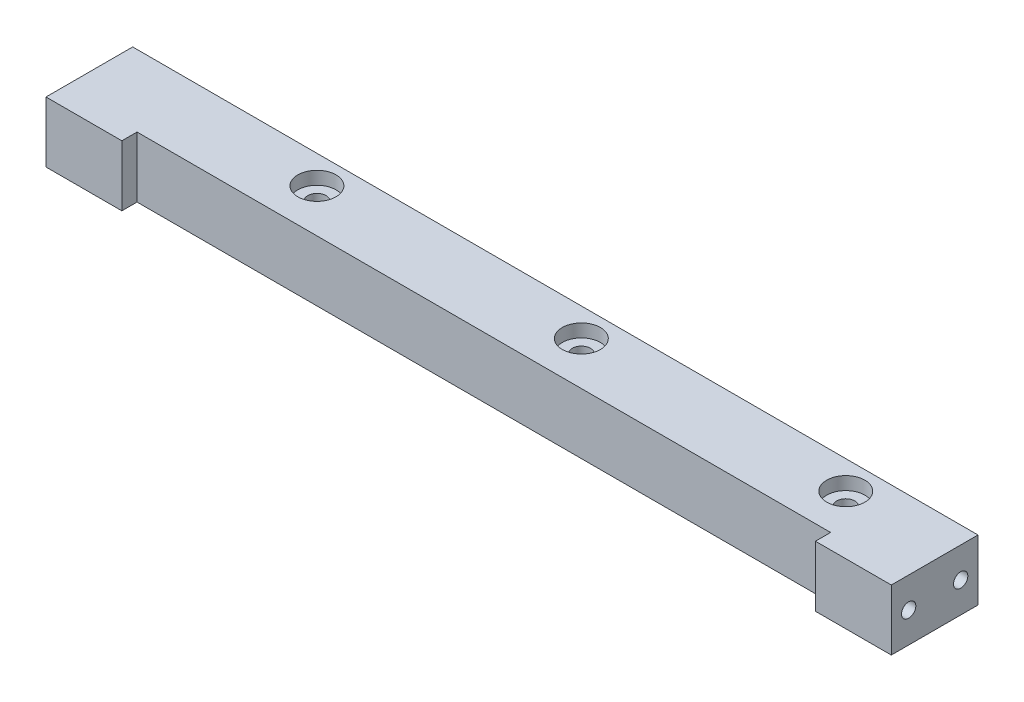
from build123d import *

# Parameters (mm, degrees)
SKETCH1_W             = 195
SKETCH1_H             = 14
EXTRUDE_THIN1_DEPTH   = 10
M4_TAPPED_HOLE1_D     = 3.3
M4_TAPPED_HOLE1_DEPTH = 10.1
M4_TAPPED_HOLE1_TIP   = 0.991420021
M4_TAPPED_HOLE2_D     = 3.3
M4_TAPPED_HOLE2_DEPTH = 10.1
M4_TAPPED_HOLE2_TIP   = 0.991420021
M5_TAPPED_HOLE1_D     = 4.2
SKETCH9_R             = 4.4
CUT_EXTRUDE1_DEPTH    = 3
SKETCH10_W            = 160
SKETCH10_H            = 3.5
CUT_EXTRUDE2_DEPTH    = 20


with BuildPart() as part:
    # Sketch1 → Extrude-Thin1 (new, symmetric)
    with BuildSketch(Plane.XY):
        with Locations((-97.5, 7)):
            Rectangle(SKETCH1_W, SKETCH1_H)
    extrude(amount=EXTRUDE_THIN1_DEPTH, both=True)

    # M4 Tapped Hole1
    with Locations(Plane.ZY.offset(195)):
        with Locations((-6, 7), (6, 7)):
            Hole(M4_TAPPED_HOLE1_D / 2, depth=M4_TAPPED_HOLE1_DEPTH)
            with Locations((0, 0, -(M4_TAPPED_HOLE1_DEPTH + M4_TAPPED_HOLE1_TIP / 2))):  # 118° drill point
                Cone(0, M4_TAPPED_HOLE1_D / 2, M4_TAPPED_HOLE1_TIP, mode=Mode.SUBTRACT)

    # M4 Tapped Hole2
    with Locations(Plane(origin=(0, 0, 0), x_dir=(0, 0, -1), z_dir=(1, 0, 0))):
        with Locations((-6, 7), (6, 7)):
            Hole(M4_TAPPED_HOLE2_D / 2, depth=M4_TAPPED_HOLE2_DEPTH)
            with Locations((0, 0, -(M4_TAPPED_HOLE2_DEPTH + M4_TAPPED_HOLE2_TIP / 2))):  # 118° drill point
                Cone(0, M4_TAPPED_HOLE2_D / 2, M4_TAPPED_HOLE2_TIP, mode=Mode.SUBTRACT)

    # M5 Tapped Hole1 (through all)
    with Locations(Plane(origin=(0, 14, 0), x_dir=(1, 0, 0), z_dir=(0, 1, 0))):
        with Locations((-146, 3.5), (-85, 3.5), (-24, 3.5)):
            Hole(M5_TAPPED_HOLE1_D / 2)

    # Sketch9 → Cut-Extrude1 (cut)
    with BuildSketch(Plane(origin=(0, 14, 0), x_dir=(1, 0, 0), z_dir=(0, 1, 0))):
        with Locations(Location((-146, 3.5, 0), (0, 0, 180))):
            Circle(SKETCH9_R)
        with Locations(Location((-85, 3.5, 0), (0, 0, 180))):
            Circle(SKETCH9_R)
        with Locations(Location((-24, 3.5, 0), (0, 0, 180))):
            Circle(SKETCH9_R)
    extrude(amount=-CUT_EXTRUDE1_DEPTH, mode=Mode.SUBTRACT)

    # Sketch10 → Cut-Extrude2 (cut)
    with BuildSketch(Plane(origin=(0, 14, 0), x_dir=(1, 0, 0), z_dir=(0, 1, 0))):
        with Locations((-97.5, -8.25)):
            Rectangle(SKETCH10_W, SKETCH10_H)
    extrude(amount=-CUT_EXTRUDE2_DEPTH, mode=Mode.SUBTRACT)


solid = part.part
